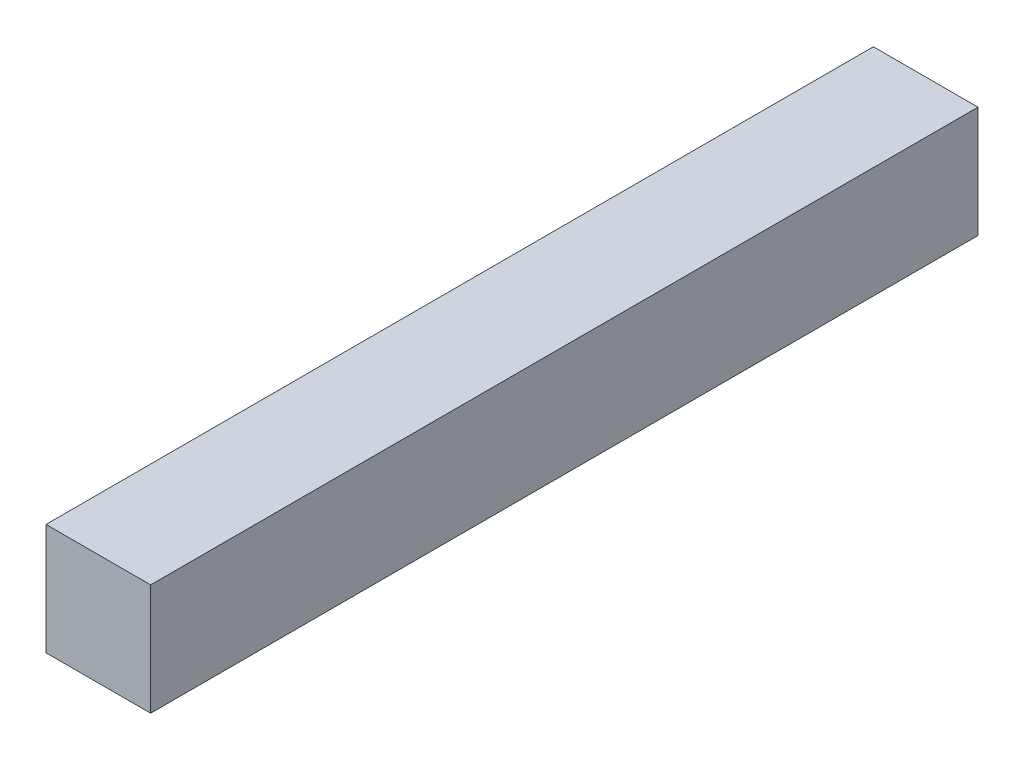
from build123d import *

# Parameters (mm, degrees)
SKETCH_1_W      = 32
SKETCH_1_H      = 34
EXTRUDE_1_DEPTH = 253


with BuildPart() as part:
    # 草图1 → 凸台-拉伸1 (new body)
    with BuildSketch(Plane.XY):
        Rectangle(SKETCH_1_W, SKETCH_1_H)
    extrude(amount=EXTRUDE_1_DEPTH)


solid = part.part
